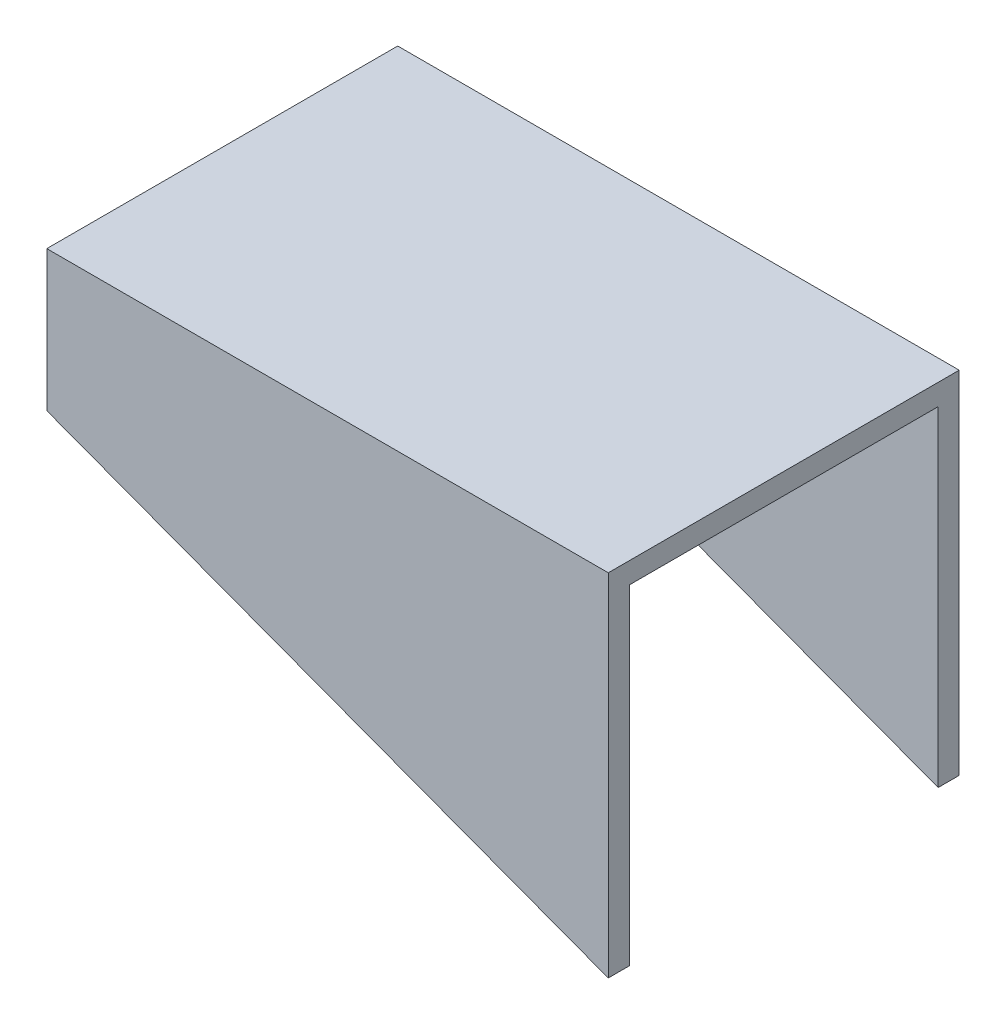
SolidWorks part; units mm, degrees
ref_plane "前视基准面" through (0, 0, 0) normal (0, 0, 1) x (1, 0, 0)
ref_plane "上视基准面" through (0, 0, 0) normal (0, 1, 0) x (1, 0, 0)
ref_plane "右视基准面" through (0, 0, 0) normal (1, 0, 0) x (0, 0, -1)
sketch "草图1" plane through (0, 0, 0) normal (0, 0, 1) x (1, 0, 0)
  line L0 (0, 0) -> (0, 50)
  line L1 (0, 50) -> (-80, 50)
  line L2 (-80, 50) -> (-80, 30)
  line L3 (-80, 30) -> (0, 0)
extrude "凸台-拉伸1" add sketch "草图1" along normal blind 50
shell "抽壳1" thickness 3
